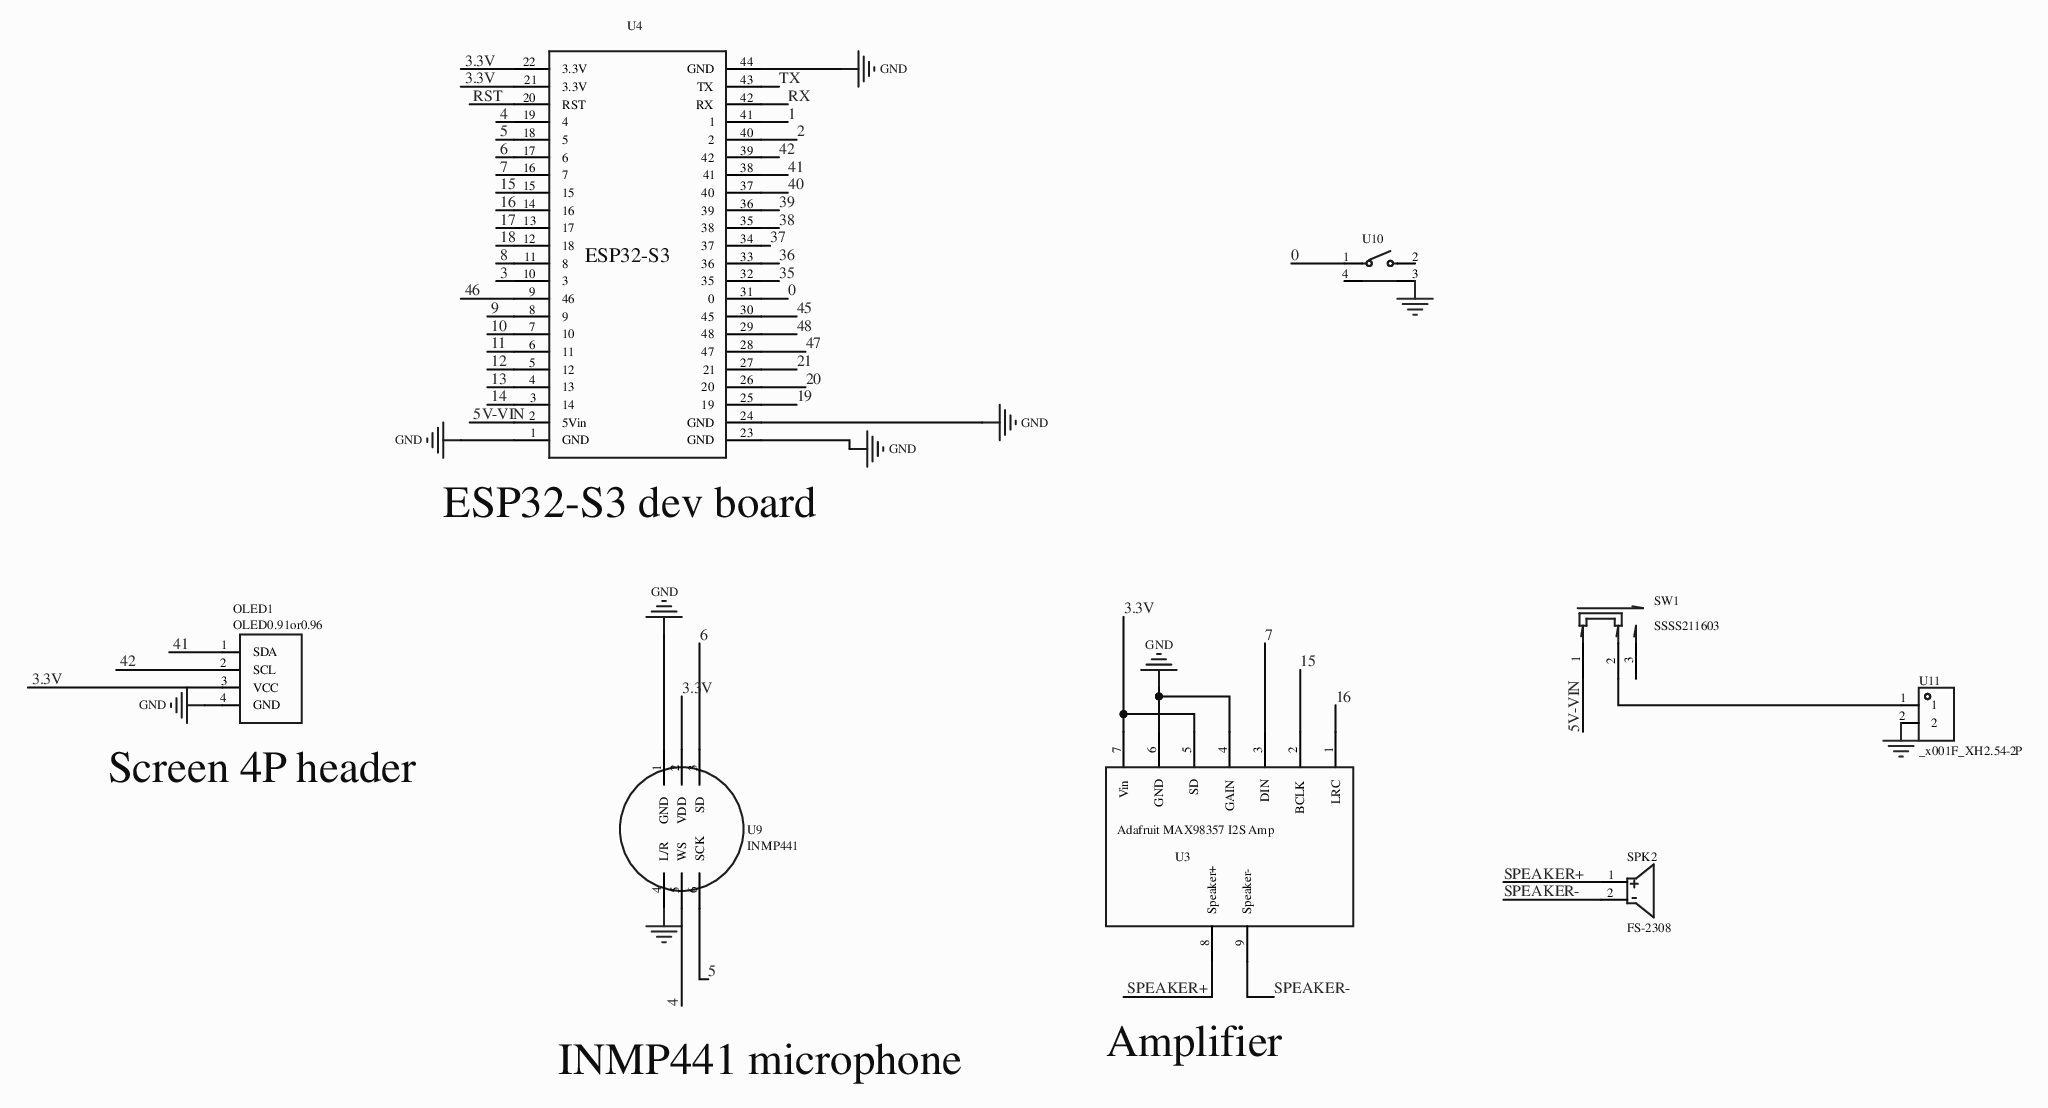
[diagram p0: MISC49945-3.schdoc]
# Altium project MISC49945-2.PrjPcb
1 sheet, 8 parts. Net scope: global (net labels, ports and power ports of the same name join across sheets).
Board file: MISC49945.pcbdoc

## Sheet MISC49945-3.schdoc
size 505 x 505 mm; Name: MISC49945; @Project Name: MISC49945; REV: 1.0; Date: 2025-01-24; Sheet: 1/1; @Page No: 1; @Page Count: 1; @Schematic Name: MISC49945; @Board Name: MISC49945; @Update Date: 2026-04-19; @Create Time: 13:59:00; @Update Time: 16:32:12; @Create Date: 2026-04-19

### Parts
OLED1  OLED0.91or0.96  [OLED0.91]
SPK2  FS-2308  [BEEP-TH_BD23.2-P9.20-D1.0]
SW1  SSSS211603  [SW-SMD_SSSS211603]
U3  Adafruit MAX98357 I2S Amp  [MAX98357 I2S AMP MODULE]
U4  NO  [ESP32S3]  (value not drawn)
U9  INMP441  [INMP441]
U10  GT-TC054A-H038-L1  [SW-SMD_L7.8-W3.5-P4.20-EH]  (value not drawn)
U11  _x001F_XH2.54-2P  [CONN-TH_2P-P2.54-V]

### Nets
GND: OLED1.4(GND) U3.4(GAIN) U3.6(GND) U4.1(GND) U4.23(GND) U4.24(GND) U4.44(GND) U9.1(GND) U9.4(L/R) U10.3 U11.2
0: U4.31(0) U10.1
1: U4.41(1)
2: U4.40(2)
3: U4.10(3)
3.3V: OLED1.3(VCC) U3.5(SD) U3.7(Vin) U4.21(3.3V) U4.22(3.3V) U9.2(VDD)
4: U4.19(4) U9.5(WS)
5: U4.18(5) U9.6(SCK)
5V-VIN: SW1.1 U4.2(5Vin)
6: U4.17(6) U9.3(SD)
7: U3.3(DIN) U4.16(7)
8: U4.11(8)
9: U4.8(9)
10: U4.7(10)
11: U4.6(11)
12: U4.5(12)
13: U4.4(13)
14: U4.3(14)
15: U3.2(BCLK) U4.15
16: U3.1(LRC) U4.14(16)
17: U4.13(17)
18: U4.12(18)
19: U4.25(19)
20: U4.26(20)
21: U4.27(21)
35: U4.32(35)
36: U4.33(36)
37: U4.34(37)
38: U4.35(38)
39: U4.36(39)
40: U4.37(40)
41: OLED1.1(SDA) U4.38(41)
42: OLED1.2(SCL) U4.39(42)
45: U4.30(45)
46: U4.9(46)
47: U4.28(47)
48: U4.29(48)
RST: U4.20(RST)
RX: U4.42(RX)
SPEAKER+: SPK2.1 U3.8(Speaker+)
SPEAKER-: SPK2.2 U3.9(Speaker-)
TX: U4.43(TX)
NetSW1_2: SW1.2 U11.1

Not connected (* = marked no-connect by the designer): SW1 3; U10 2 4

### Notes on the sheet
- (near U4) ESP32-S3 dev board
- (near OLED1) Screen 4P header
- INMP441 microphone
- Amplifier

### Library data of the parts
OLED1 = OLED0.91or0.96: Convert to PCB: yes; Origin Footprint: OLED0.91; Device: OLED0.91or0.96; Symbol: OLED0.91or0.96; Add into BOM: yes; FootprintName: OLED0.91
SPK2 = FS-2308: Manufacturer: FUET(福声科技); Add into BOM: yes; ModelId: f2de6d3d53f440b38eb7d42236cfa69c; ModelTransform: 905.51,905.51,0,90,0,0,0,0,-118.11; Symbol: FS-2308; Device: FS-2308; LCSC Part Name: 喇叭23MM-8.0H 8Ω1W 插针; SupplierPart: C482322; ManufacturerPart: FS-2308; Supplier Footprint: -; JLCPCB Part Class: Extended library; Datasheet: example.com/20200113/C482322_D09CD61BAFBB8D4AD64070E01BFD18FF.pdf; Supplier: LCSC; ConvertToPcb: yes; FootprintName: BEEP-TH_BD23.2-P9.20-D1.0; ModelName: BEEP-TH_BD23.2-P9.20-D1.0
SW1 = SSSS211603: Circuit: SPDT; mounting: horizontal (SMD); rated current (DC): 300mA; rated voltage (DC): 6V; rated current (AC): -; rated voltage (AC): -; mechanical life: 1万 cycles;; Manufacturer: ALPSALPINE(阿尔卑斯阿尔派); Add into BOM: yes; ModelId: 3a2e49b97cce4d39aea5f9c64a29d8f7; ModelTransform: 354.33,295.275,0,180,0,0,1.142,108.819,0; Actuator Style: Rectangular post; Pin Style: SMD tab; Switch Height: 5.5mm; Symbol: SSSS211603; Device: SSSS211603; LCSC Part Name: 8.5*3.5*3.5 立式、侧滑; SupplierPart: C125040; ManufacturerPart: SSSS211603; Supplier Footprint: SMD; JLCPCB Part Class: Extended library; Datasheet: example.com/20170810/C125040_1502335339949879900.pdf; Supplier: LCSC; ConvertToPcb: yes; FootprintName: SW-SMD_SSSS211603; ModelName: SW-SMD_SSSS211603; Mounting Style: Horizontal SMD; Current Rating (DC): 300mA; Voltage Rating (DC): 6V; Current Rating (AC): -; Voltage Rating (AC): -; Mechanical Life: 1万 cycles; Operating Temperature: -40℃~+85℃
U3 = Adafruit MAX98357 I2S Amp: Convert to PCB: yes; Origin Footprint: MAX98357 I2S AMP MODULE; Device: Adafruit MAX98357 I2S Amp; Symbol: Adafruit MAX98357 I2S Amp; Manufacturer Part: Adafruit MAX98357 I2S Amp; Add into BOM: yes; FootprintName: MAX98357 I2S AMP MODULE
U4 = NO: Convert to PCB: yes; Origin Footprint: ESP32S3; Device: NO; Symbol: NO; Add into BOM: yes; FootprintName: ESP32S3
U9 = INMP441: Convert to PCB: yes; Origin Footprint: INMP441; Device: INMP441; Symbol: INMP441; Add into BOM: yes; FootprintName: INMP441
U10 = GT-TC054A-H038-L1: Circuit: SPST; actuating force: 1.6N; mounting: -; with bracket: no; contact current: 50mA; rated voltage (AC): 12V; rated voltage (DC): 12V; insulation resistance: 100MΩ; with lamp: no; mechanical life: 10万 cycles;; Manufacturer: G-Switch(品赞); Add into BOM: yes; ModelId: ee81f3e065e84f458ab74fe15f8d856e; ModelName: SW-SMD_L7.8-W3.5-H3.5-P4.20-EH; ModelTransform: 307.086,157.48,0,0,0,0,0,17.48,-31.496; Strike Gundam: Without; With Lamp: None; Symbol: GT-TC054A-H038-L1; Device: GT-TC054A-H038-L1; LCSC Part Name: 3*6侧按轻触开关 H3.8 180gf; SupplierPart: C19188077; ManufacturerPart: GT-TC054A-H038-L1; Supplier Footprint: SMD,7.8x3.6mm,侧贴; JLCPCB Part Class: Extended library; Datasheet: example.com/20231127/BB860A649B8AA9AECA1C37B9D3F71741.pdf; Supplier: LCSC; ConvertToPcb: yes; FootprintName: SW-SMD_L7.8-W3.5-P4.20-EH; Operating Force: 1.6N; Mounting Style: -; Contact Current: 50mA; Voltage Rating (AC): 12V; Voltage Rating (DC): 12V; Insulation Resistance: 100MΩ; Mechanical Life: 10万 cycles
U11 = _x001F_XH2.54-2P: Add into BOM: yes; ModelId: 4b619f877c224111ac90f050b36c3583; ModelTransform: 295.275,224.409,0,180,0,0,0,17.717,-118.11; Symbol: _X001F_XH2.54-2P; Device: _x001F_XH2.54-2P; LCSC Part Name: _x001F_XH2.54-2P; SupplierPart: C9900016027; ManufacturerPart: _x001F_XH2.54-2P; Supplier Footprint: XH2.54-2P直插; JLCPCB Part Class: Extended library; Supplier: LCSC; ConvertToPcb: yes; FootprintName: CONN-TH_2P-P2.54-V; ModelName: CONN-TH_2P-P2.54-V